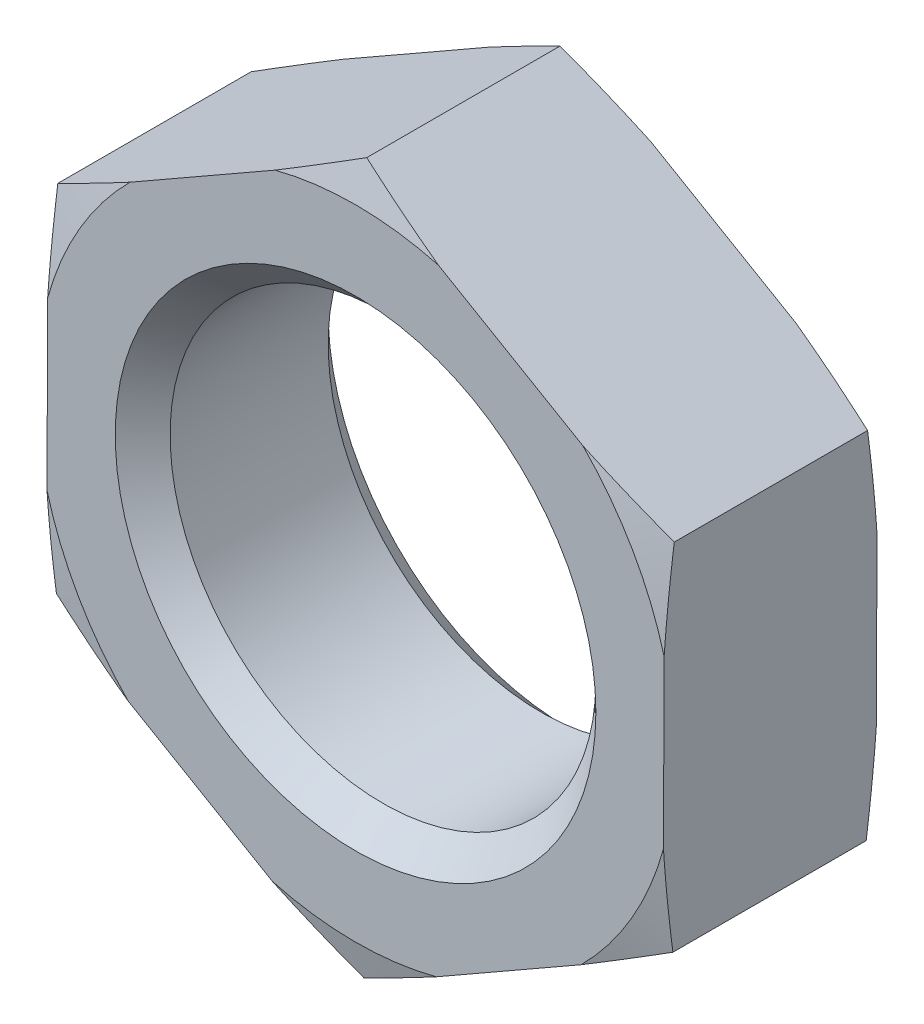
SolidWorks part; units mm, degrees
extrude "基体-拉伸" add sketch "草图1" along normal blind 8
sketch "草图1" plane through (0, 0, 0) normal (0, 0, 1) x (1, 0, 0)
  line L0 (-26.8088, 0) -> (37.1748, 0) construction
  line L1 (0, 25.0215) -> (0, -25.0215) construction
  line L3 (0.0526, 13.3749) -> (-11.5567, 6.733)
  line L4 (-11.5567, 6.733) -> (-11.6093, -6.6419)
  line L5 (-11.6093, -6.6419) -> (-0.0526, -13.3749)
  line L6 (-0.0526, -13.3749) -> (11.5567, -6.733)
  line L7 (11.5567, -6.733) -> (11.6093, 6.6419)
  line L8 (11.6093, 6.6419) -> (0.0526, 13.3749)
  circle A0 centre (0, 0) radius 11.5831 construction
  circle A1 centre (0, 0) radius 8
cosmetic thread "装饰螺纹线1"
chamfer "倒角1" distance 1.031 angle 45 2 edges at (8, 0, 0) (8, 0, 8)
material "04级"
ref_plane "基准面1" through (0, 0, 0) normal (0, 0, 1) x (1, 0, 0)
ref_plane "基准面2" through (0, 0, 0) normal (0, 1, 0) x (1, 0, 0)
ref_plane "基准面3" through (0, 0, 0) normal (1, 0, 0) x (0, 0, -1)
sketch "尺寸草图" plane through (0, 0, 0) normal (0, 0, 1) x (1, 0, 0)
  line L0 (0, 0) -> (24.1005, 0)
  line L1 (27.4249, 65.7219) -> (44.7249, 65.7219)
  line L2 (46.8781, 65.7219) -> (69.3781, 65.7219)
  line L3 (-37.8187, 0) -> (-22.5806, 0)
  point P3 (16, 0)
  point P4 (1.5, 0)
  point P5 (26.75, 0)
  point P6 (8, 0)
  point P7 (24.32, 0)
  point P8 (24, 0)
sketch "草图2" plane through (0, 0, 0) normal (0, 0, -1) x (-1, 0, 0)
  circle A0 centre (0, 0) radius 12
  circle A1 centre (0, 0) radius 8 construction
extrude "切除-拉伸1" cut sketch "草图2" against normal through all draft 75 flip side to cut
sketch "草图3" plane through (0, 0, 8) normal (0, 0, 1) x (1, 0, 0)
  circle A0 centre (0, 0) radius 12
extrude "切除-拉伸2" cut sketch "草图3" against normal through all draft 75 flip side to cut
equation "\"e@草图1\" = \"e@尺寸草图\""
equation "\"D1@尺寸草图\" = \"D@尺寸草图\" / 1.05"
equation "\"D@草图1\" = \"D@尺寸草图\""
equation "\"m@基体-拉伸\" = \"m@尺寸草图\""
equation "\"D1@草图3\" = \"s@尺寸草图\""
equation "\"s@草图2\" = \"s@尺寸草图\""
equation "\"D2@装饰螺纹线1\" = 1.05 * \"D1@尺寸草图\""
equation "\"D1@倒角1\" =  ( \"da@尺寸草图\" - \"D1@尺寸草图\" )  / 2"
